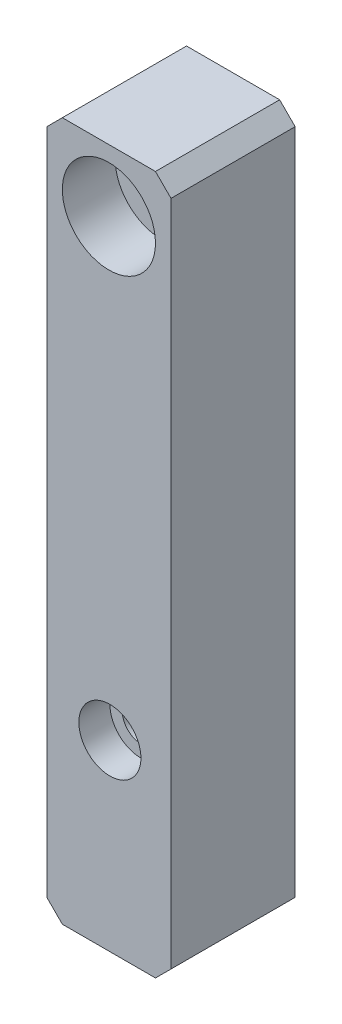
from build123d import *

# Parameters (mm, degrees)
SKETCH1_W                                           = 8
SKETCH1_H                                           = 45
BOSS_EXTRUDE1_DEPTH                                 = 8
HOLE_SIZE_PER_SOCKET_HEAD_CAP_SCREW_TYP_D           = 3.4
HOLE_SIZE_PER_SOCKET_HEAD_CAP_SCREW_TYP_CBORE_D     = 6
HOLE_SIZE_PER_SOCKET_HEAD_CAP_SCREW_TYP_CBORE_DEPTH = 3.4
SKETCH2_R                                           = 2
CUT_EXTRUDE1_DEPTH                                  = 2
HOLE_SIZE_PER_SOCKET_HEAD_CAP_SCREW_2_D             = 2.4
HOLE_SIZE_PER_SOCKET_HEAD_CAP_SCREW_2_CBORE_D       = 4.3
HOLE_SIZE_PER_SOCKET_HEAD_CAP_SCREW_2_CBORE_DEPTH   = 2.3
CHAMFER1_SIZE                                       = 1


with BuildPart() as part:
    # Sketch1 → Boss-Extrude1 (new body)
    with BuildSketch(Plane.XY):
        with Locations((-10.344506296, -27.5)):
            Rectangle(SKETCH1_W, SKETCH1_H)
    extrude(amount=BOSS_EXTRUDE1_DEPTH)

    # Hole size _per socket head cap screw typ (through all)
    with Locations(Plane(origin=(-10.344506296, -9, 8), x_dir=(1, 0, 0), z_dir=(0, 0, 1))):
        with Locations((0, 0)):
            CounterBoreHole(HOLE_SIZE_PER_SOCKET_HEAD_CAP_SCREW_TYP_D / 2, HOLE_SIZE_PER_SOCKET_HEAD_CAP_SCREW_TYP_CBORE_D / 2, HOLE_SIZE_PER_SOCKET_HEAD_CAP_SCREW_TYP_CBORE_DEPTH)

    # Sketch2 → Cut-Extrude1 (cut)
    with BuildSketch(Plane.XY.offset(8)):
        with Locations((-10.281246694, -38.2)):
            Circle(SKETCH2_R)
    extrude(amount=-CUT_EXTRUDE1_DEPTH, mode=Mode.SUBTRACT)

    # Hole size _per socket head cap screw 2 (through all)
    with Locations(Plane(origin=(-10.281246694, -38.2, 0), x_dir=(-1, 0, 0), z_dir=(0, 0, -1))):
        with Locations((0, 0)):
            CounterBoreHole(HOLE_SIZE_PER_SOCKET_HEAD_CAP_SCREW_2_D / 2, HOLE_SIZE_PER_SOCKET_HEAD_CAP_SCREW_2_CBORE_D / 2, HOLE_SIZE_PER_SOCKET_HEAD_CAP_SCREW_2_CBORE_DEPTH)

    # Chamfer1
    chamfer1_edges = [part.edges().sort_by_distance(p)[0] for p in [
        (-14.344506296, -5, 4),
        (-14.344506296, -50, 4),
        (-6.344506296, -50, 4),
        (-6.344506296, -5, 4),
    ]]
    chamfer(chamfer1_edges, length=CHAMFER1_SIZE)


solid = part.part
